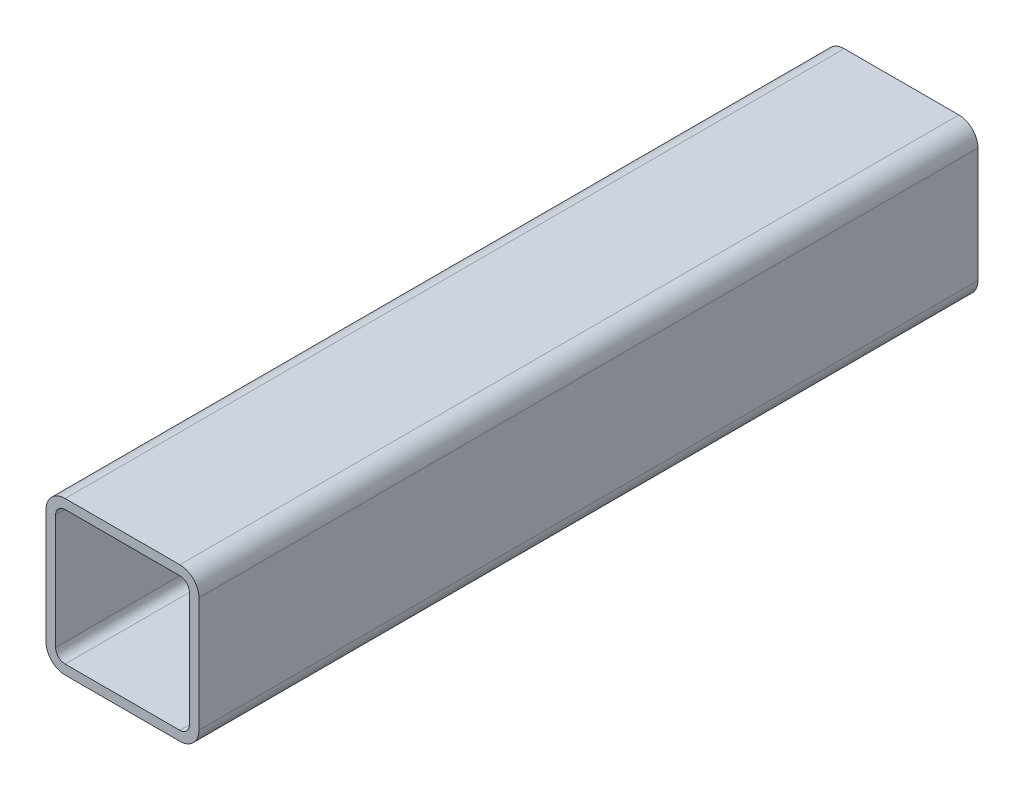
from build123d import *

# Parameters (mm, degrees)
BOSS_EXTRUDE_1_DEPTH = 163


with BuildPart() as part:
    # Sketch 1 → Boss-Extrude 1 (new, symmetric)
    with BuildSketch(Plane.XY):
        with BuildLine():
            Line((0, 32), (-24, 32))
            ThreePointArc((-24, 32), (-29.656854249, 29.656854249), (-32, 24))
            Line((-32, 24), (-32, 0))
            Line((-32, 0), (-32, -24))
            ThreePointArc((-32, -24), (-29.656854249, -29.656854249), (-24, -32))
            Line((-24, -32), (24, -32))
            ThreePointArc((24, -32), (29.656854249, -29.656854249), (32, -24))
            Line((32, -24), (32, 0))
            Line((32, 0), (32, 24))
            ThreePointArc((32, 24), (29.656854249, 29.656854249), (24, 32))
            Line((24, 32), (0, 32))
        make_face()
        with BuildLine():
            Line((0, 28), (-24, 28))
            ThreePointArc((-24, 28), (-26.828427125, 26.828427125), (-28, 24))
            Line((-28, 24), (-28, 0))
            Line((-28, 0), (-28, -24))
            ThreePointArc((-28, -24), (-26.828427125, -26.828427125), (-24, -28))
            Line((-24, -28), (24, -28))
            ThreePointArc((24, -28), (26.828427125, -26.828427125), (28, -24))
            Line((28, -24), (28, 0))
            Line((28, 0), (28, 24))
            ThreePointArc((28, 24), (26.828427125, 26.828427125), (24, 28))
            Line((24, 28), (0, 28))
        make_face(mode=Mode.SUBTRACT)
    extrude(amount=BOSS_EXTRUDE_1_DEPTH, both=True)


solid = part.part
